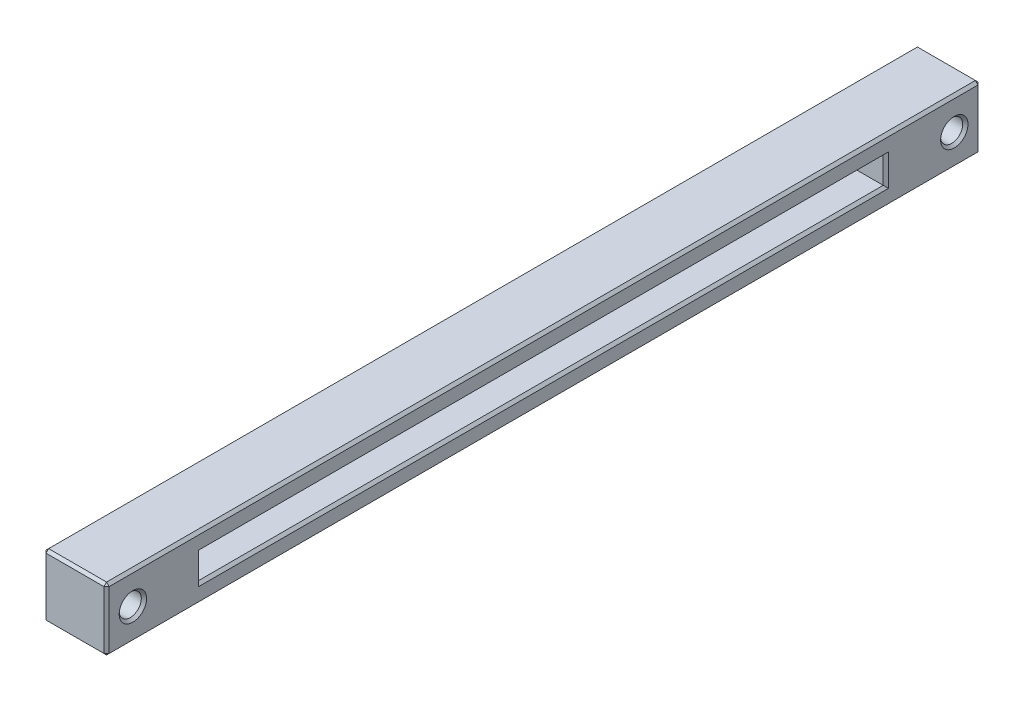
SolidWorks part; units mm, degrees
ref_plane "前视基准面" through (0, 0, 0) normal (0, 0, 1) x (1, 0, 0)
ref_plane "上视基准面" through (0, 0, 0) normal (0, 1, 0) x (1, 0, 0)
ref_plane "右视基准面" through (0, 0, 0) normal (1, 0, 0) x (0, 0, -1)
sketch "草图1" plane through (0, 0, 0) normal (1, 0, 0) x (0, 0, -1)
  line L1 (-830, 60) -> (830, 60)
  line L2 (-830, 60) -> (-830, -60)
  line L3 (-830, -60) -> (830, -60)
  line L4 (830, 60) -> (830, -60)
  line L5 (-830, 60) -> (830, -60) construction
  line L6 (-830, -60) -> (830, 60) construction
  point P0 (0, 0)
  dimension "D1" = 1660
  dimension "D2" = 120
extrude "凸台-拉伸1" add sketch "草图1" along normal blind 120
sketch "草图2" plane through (120, 0, 0) normal (1, 0, 0) x (0, 0, -1)
  line L1 (-650, 25) -> (650, 25)
  line L2 (-650, 25) -> (-650, -25)
  line L3 (-650, -25) -> (650, -25)
  line L4 (650, 25) -> (650, -25)
  line L5 (-650, 25) -> (650, -25) construction
  line L6 (-650, -25) -> (650, 25) construction
  point P0 (0, 0)
  dimension "D1" = 50
  dimension "D2" = 1300
extrude "切除-拉伸1" cut sketch "草图2" against normal through all
sketch "草图3" plane through (120, 0, 0) normal (1, 0, 0) x (0, 0, -1)
  line L0 (0, -60) -> (0, 378.3221) construction
  line L1 (-830, -60) -> (830, -60) construction
  line L2 (-830, 0) -> (-417.295, 0) construction
  line L3 (-830, 60) -> (-830, -60) construction
  circle A0 centre (-780, 0) radius 21
  circle A1 centre (780, 0) radius 21
  dimension "D2" = 42
  dimension "D1" = 1560
extrude "切除-拉伸2" cut sketch "草图3" against normal through all
chamfer "倒角1" distance 5 angle 45 24 edges at (120, 25, 0) (120, 0, 650) (120, -25, 0) (120, 0, -650) (120, 0, -801) (120, 0, 759) (0, -60, 0) (0, 60, 0) (60, -60, -830) (0, 0, -830) (60, 60, -830) (120, -60, 0) (120, 0, -830) (120, 60, 0) (60, 60, 830) (120, 0, 830) (60, -60, 830) (0, 0, 830) (0, 0, 650) (0, 25, 0) (0, 0, -650) (0, -25, 0) (0, 0, -801) (0, 0, 759)
